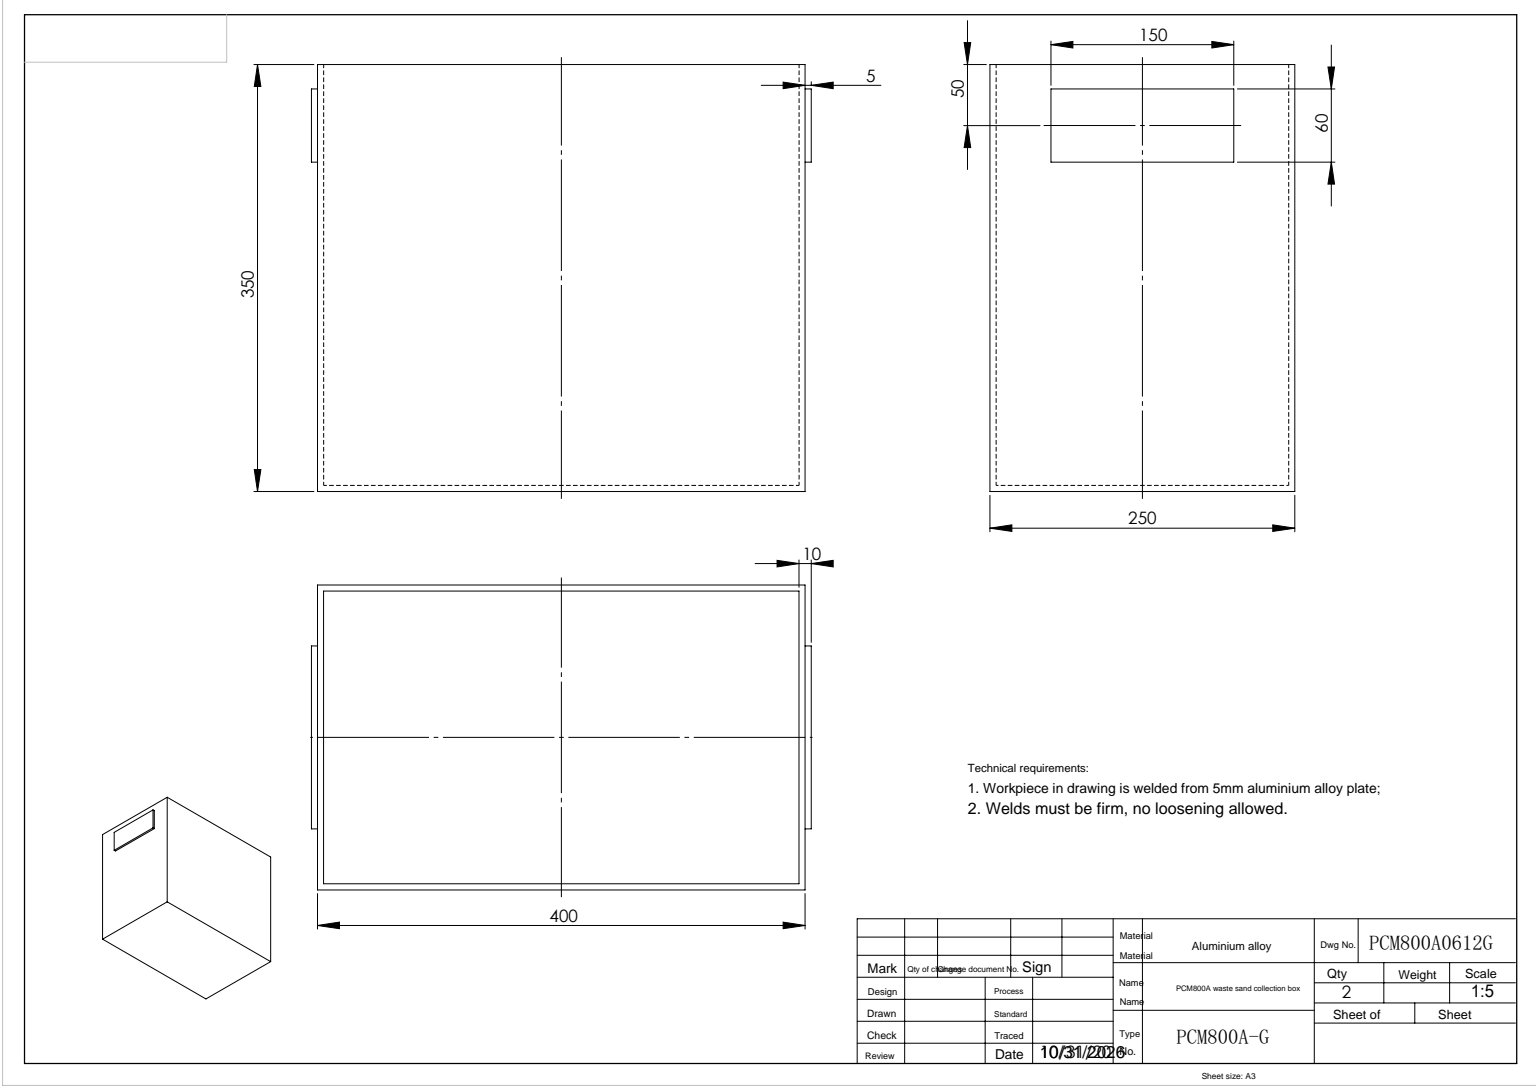
SolidWorks part; units mm, degrees
ref_plane "前视" through (0, 0, 0) normal (0, 0, 1) x (1, 0, 0)
ref_plane "上视" through (0, 0, 0) normal (0, 1, 0) x (1, 0, 0)
ref_plane "右视" through (0, 0, 0) normal (1, 0, 0) x (0, 0, -1)
sketch "草图1" plane through (0, 0, 0) normal (0, 1, 0) x (1, 0, 0)
  line L1 (0, 0) -> (400, 0)
  line L2 (0, 0) -> (0, 250)
  line L3 (0, 250) -> (400, 250)
  line L4 (400, 0) -> (400, 250)
  dimension "D1" = 400
  dimension "D2" = 250
extrude "凸台-拉伸1" add sketch "草图1" along normal blind 350
shell "抽壳1" thickness 5
sketch "草图2" plane through (400, 0, 0) normal (1, 0, 0) x (0, 0, -1)
  line L0 (125, 350) -> (125, -11.0645) construction
  line L1 (0, 350) -> (250, 350) construction
  line L3 (50, 330) -> (200, 330)
  line L4 (50, 330) -> (50, 270)
  line L5 (50, 270) -> (200, 270)
  line L6 (200, 330) -> (200, 270)
  dimension "D1" = 60
  dimension "D2" = 150
  dimension "D3" = 75
  dimension "D4" = 20
extrude "凸台-拉伸2" add sketch "草图2" along normal blind 5
sketch "草图3" plane through (0, 0, 0) normal (-1, 0, 0) x (0, 0, 1)
  line L0 (-125, 350) -> (-125, 0) construction
  line L1 (-250, 350) -> (0, 350) construction
  line L2 (-250, 0) -> (0, 0) construction
  line L4 (-200, 330) -> (-50, 330)
  line L5 (-200, 330) -> (-200, 270)
  line L6 (-200, 270) -> (-50, 270)
  line L7 (-50, 330) -> (-50, 270)
  dimension "D1" = 60
  dimension "D2" = 150
  dimension "D3" = 75
  dimension "D4" = 20
extrude "凸台-拉伸3" add sketch "草图3" along normal blind 5
